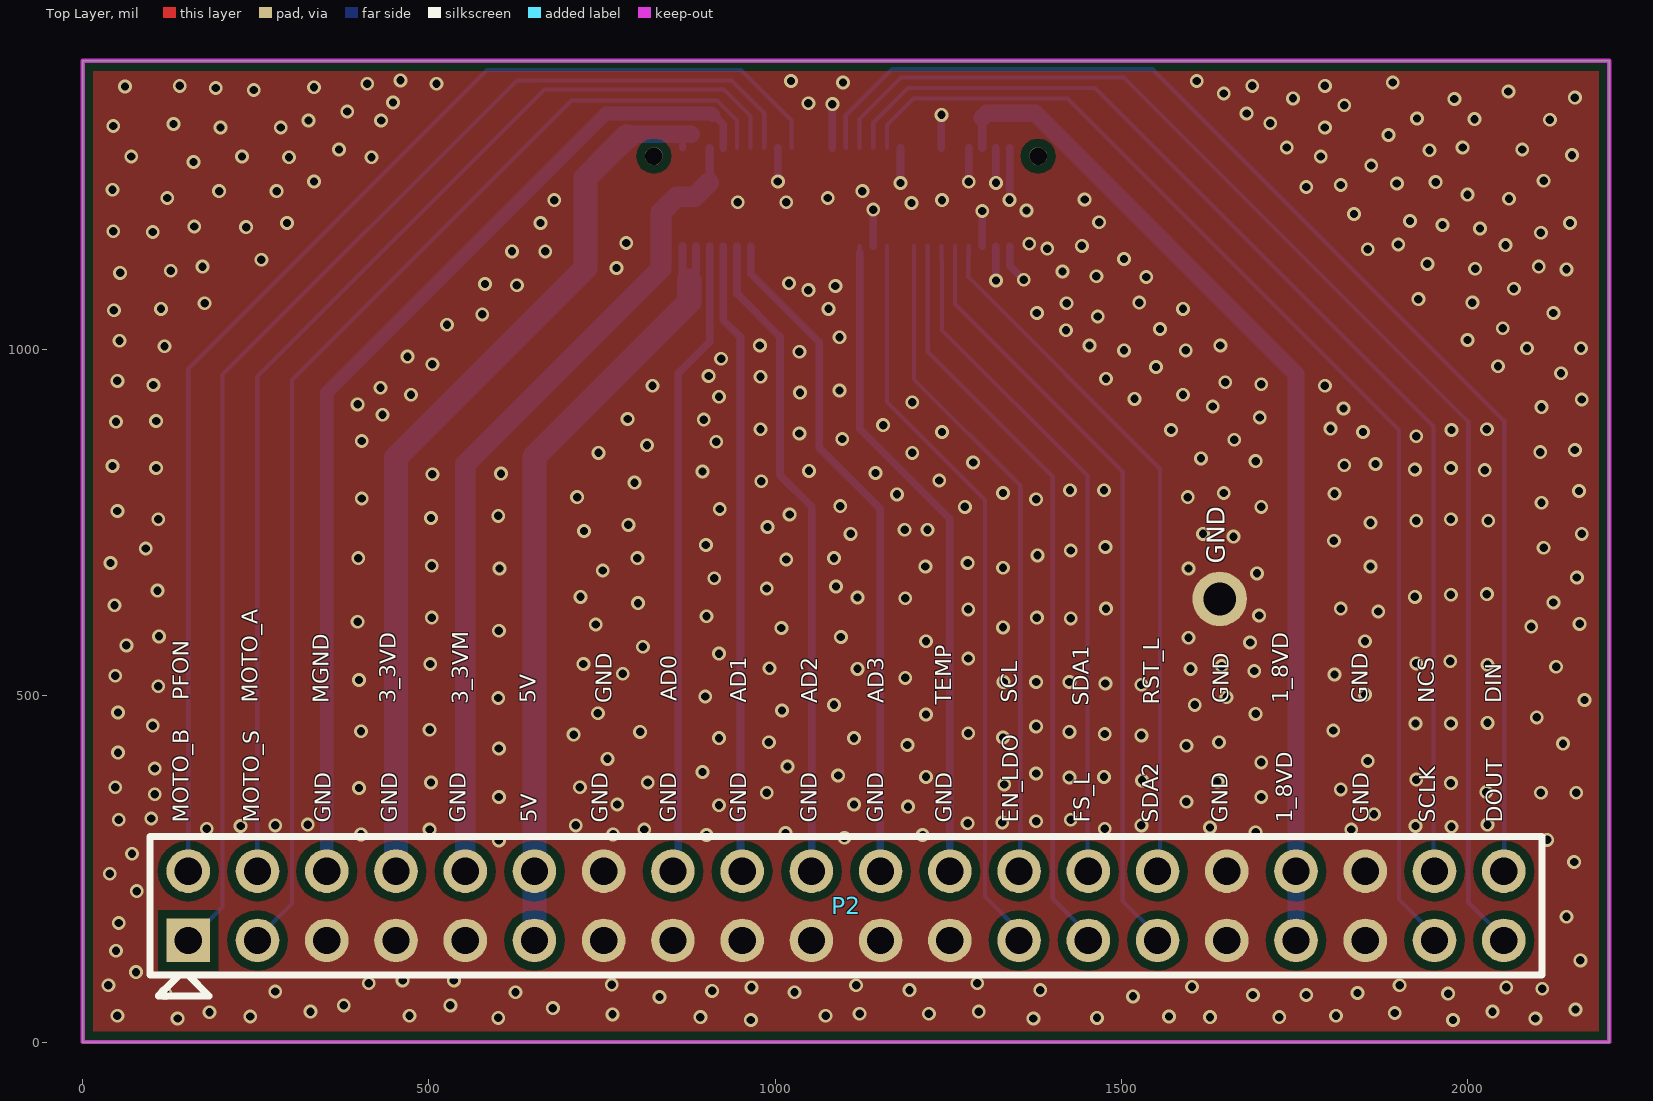
[diagram p0: Top Layer view]
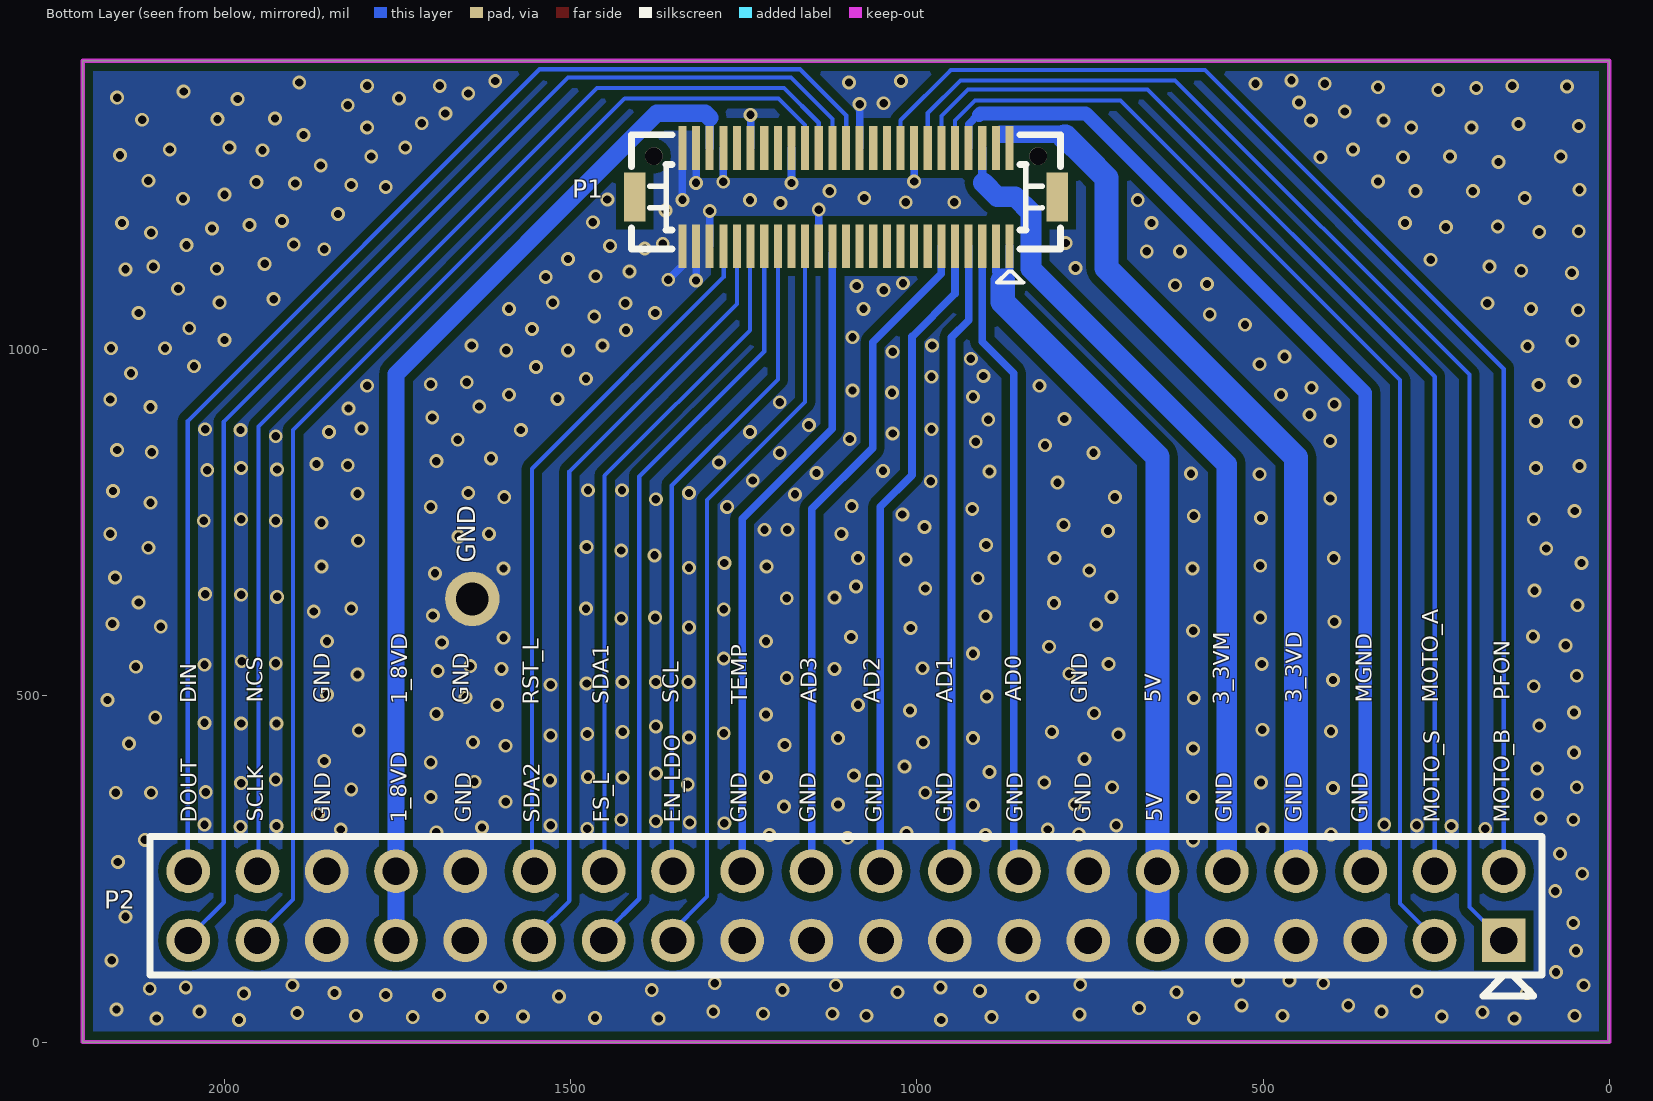
[diagram p1: Bottom Layer view, seen from below]
# Altium PCB MISC89329.PcbDoc
Units mil, origin at the board's own origin, x right, y up, seen from the top; angles counter-clockwise.
Board outline 2204.72 x 1417.32 mil, 2 copper layers (Top Layer, Bottom Layer); 2 components, 25 nets, 95 pads, 502 vias.

## Layer stack, top to bottom (the 12.6 mil dielectric is the usual default, probably not edited)
Top Layer: signal copper 1.4
Dielectric: dielectric 12.6, FR-4, Dk 4.8
Bottom Layer: signal copper 1.4

## Board outline
2204.72,1417.32 0,1417.32 0,0 2204.72,0

## Design rules (kind name [scope] priority, off if disabled: settings)
Clearance Clearance_1 [inpolygon] p1: gap=12
Clearance [All] p2: gap=6
DiffPairsRouting [All] p1: maxlimit=6 minlimit=6 mostfreqgap=6 maxuncoupledlength=500
HoleSize [All] p1: absolutevalues=TRUE maxlimit=500 minlimit=1 maxpercent=80.000 minpercent=20.000
HoleToHoleClearance [All] p1: gap=0 allowstackedmicrovias=TRUE
MinimumSolderMaskSliver [All] p1: minsoldermaskwidth=0
PlaneClearance [All] p1: clearance=6
PlaneConnect [All] p1: planeconnectstyle=Direct reliefexpansion=20 reliefentries=4 reliefconductorwidth=10 reliefairgap=10
PolygonConnect [All] p1: connectstyle=Direct reliefconductorwidth=10 reliefentries=4 polygonreliefangle="90 Angle"
RoutingVias [All] p1: holewidth=12 width=20 viastyle="Through Hole" minholewidth=12 minwidth=20 maxholewidth=12 maxwidth=20
SilkToSilkClearance [All] p1: silktosilkclearance=0
SilkscreenOverComponentPads [All] p1: minsilkscreentomaskgap=0
SolderMaskExpansion [All] p1: expansion=4
Width [All] p1: maxlimit=80 minlimit=6 preferedwidth=6 minimp=50.000000 maximp=50.000000 favimp=50.000000
20 further rules are at their usual default settings.

## Components (designator, comment, footprint, x,y, rotation, side; value= is the part's Value field where it differs from the comment)
P1 "#NAME?" CONN-SMD_DF12A-3.0-50DS-0.5 1102.36,1220.47 r180 bottom
P2 "#NAME?" HDR-TH_40P-P2.54-V-F-R2-C20-S2.54 1102.36,196.85 r0 top locked

## Footprints (in the part's own frame and the unit in brackets; to place one, negate y for a bottom-side part, rotate by r counter-clockwise, add the part's x,y. Pads: shape width x height; smd on the part's side, far side on the other; paste and mask are expansions set on the pad)
CONN-SMD_DF12A-3.0-50DS-0.5 [mm]
  round 0.65 hole 0.65 unplated: 0(-7.049,1.5) 0(7.049,1.5)
  rect 0.297x1.598 smd: 1(5.999,-1.798) 2(5.999,1.798) 3(5.499,-1.798) 4(5.499,1.798) 5(4.999,-1.798) 6(4.999,1.798) 7(4.499,-1.798) 8(4.499,1.798) 9(3.999,-1.798) 10(3.999,1.798) 11(3.499,-1.798) 12(3.499,1.798) 13(2.999,-1.798) 14(2.999,1.798) 15(2.499,-1.798) 16(2.499,1.798) 17(1.999,-1.798) 18(1.999,1.798) 19(1.499,-1.798) 20(1.499,1.798) 21(0.999,-1.798) 22(0.999,1.798) 23(0.499,-1.798) 24(0.499,1.798) 25(-0.001,-1.798) 26(-0.001,1.798) 27(-0.501,-1.798) 28(-0.501,1.798) 29(-1.001,-1.798) 30(-1.001,1.798) 31(-1.501,-1.798) 32(-1.501,1.798) 33(-2.001,-1.798) 34(-2.001,1.798) 35(-2.501,-1.798) 36(-2.501,1.798) 37(-3.001,-1.798) 38(-3.001,1.798) 39(-3.501,-1.798) 40(-3.501,1.798) 41(-4.001,-1.798) 42(-4.001,1.798) 43(-4.501,-1.798) 44(-4.501,1.798) 45(-5.001,-1.798) 46(-5.001,1.798) 47(-5.501,-1.798) 48(-5.501,1.798) 49(-6.001,-1.798) 50(-6.001,1.798)
  rect 0.798x1.796 smd: 51(-7.75,-0.003) 52(7.75,-0.003)
  silkscreen extent -7.87,-3.14 7.87,2.29
HDR-TH_40P-P2.54-V-F-R2-C20-S2.54 [mm]
  rect 1.6x1.6 hole 1: 1(-24.13,-1.27)
  round 1.6 hole 1: 2(-24.13,1.27) 3(-21.59,-1.27) 4(-21.59,1.27) 5(-19.05,-1.27) 6(-19.05,1.27) 7(-16.51,-1.27) 8(-16.51,1.27) 9(-13.97,-1.27) 10(-13.97,1.27) 11(-11.43,-1.27) 12(-11.43,1.27) 13(-8.89,-1.27) 14(-8.89,1.27) 15(-6.35,-1.27) 16(-6.35,1.27) 17(-3.81,-1.27) 18(-3.81,1.27) 19(-1.27,-1.27) 20(-1.27,1.27) 21(1.27,-1.27) 22(1.27,1.27) 23(3.81,-1.27) 24(3.81,1.27) 25(6.35,-1.27) 26(6.35,1.27) 27(8.89,-1.27) 28(8.89,1.27) 29(11.43,-1.27) 30(11.43,1.27) 31(13.97,-1.27) 32(13.97,1.27) 33(16.51,-1.27) 34(16.51,1.27) 35(19.05,-1.27) 36(19.05,1.27) 37(21.59,-1.27) 38(21.59,1.27) 39(24.13,-1.27) 40(24.13,1.27)
  silkscreen extent -25.53,-3.31 25.53,2.54

## Part data
P1: library part DF12A-50DS-0.5V(81)
P2: library part 2.54-2*20

## Free pads (board coordinates)
  round 78.74 hole 47.24: 0(1642,640)

## Via types
v1: diameter 20, hole 12, Top Layer to Bottom Layer, tented both sides, 502 vias

## Nets (pads, with @x,y where several pads share a name; then routed paths per layer and width w, separated by ;. In a path a pad name is that pad's centre, name@x,y a point inside that pad or via, vN(x,y) a via of type N, cw(c..) or ccw(c..) an arc to the next point about the centre after c; other vN are vias at no path point)
1_8VD: P1.46 P2.33 P2.34 | length 1470.2
  Bottom Layer w12: P1.46 1299.23,1328.77
  Bottom Layer w20: 1299.23,1331.51 1299.23,1333.23 1300.14,1334.14
  Bottom Layer w25: 1299.23,1335.05 1305.68,1341.5 1375.5,1341.5 1752.36,964.64 P2.34 P2.33
3_3VD: P1.2 P1.4 P2.8 | length 1327.6
  Bottom Layer w10: P1.2 P1.2@866.16,1311.84
  Bottom Layer w25: 794,1311 879,1311
  Bottom Layer w35: P2.8 452.36,844.36 726,1118 726,1248 755.5,1277.5 ; 771,1293 755.5,1277.5 ; 787,1307.5 785.5,1307.5 755.5,1277.5
3_3VM: P1.6 P2.10 | length 1205.4
  Bottom Layer w12: 905.53,1244.53 P1.6
  Bottom Layer w20: 903,1242 905.53,1244.53
  Bottom Layer w30: P2.10 552.36,834.36 835,1117 835,1198 858,1221 884,1221 904,1241
5V: P1.1 P1.3 P2.11 P2.12 | length 1149.9
  Bottom Layer w12: P1.1 866.16,1110.84 875,1102 ; 876,1103 885.85,1112.85 P1.3
  Bottom Layer w30: 875,1100 875,1102
  Bottom Layer w35: P2.11 P2.12 652.36,845.36 876,1069 876,1100
AD0: P1.5 P2.16 | length 901.5
  Bottom Layer w11: P2.16@860,267 860,966 905.53,1011.53 P1.5
AD1: P1.7 P2.18 | length 893.9
  Bottom Layer w11: P1.7 925.22,1042.78 950,1018 P2.18@950,266
AD2: P1.9 P2.20 | length 927.4
  Bottom Layer w11: 944.9,1095 P1.9 ; 945,1095 945,1081 1007,1019 1007,819 1053,773 P2.20@1053,267
AD3: P1.11 P2.22 | length 957.1
  Bottom Layer w11: P1.11@964.59,1128 P1.11 ; P1.11@965,1128 965,1110 1064,1011 1064,858 1152,770 P2.22@1152,270
DIN: P1.26 P2.40 | length 1942.1
  Bottom Layer w6: P1.26 1102,1291.66 1102,1338 1169,1405 1545,1405 2053,897 2053,356 ; P2.40@2053,259 2053,356 ; 2053,288 2053,356
DOUT: P1.28 P2.39 | length 1913.3
  Bottom Layer w6: P1.28 1122.07,1333.07 1182,1393 1504,1393 2001,896 2001,202 P2.39@2049,154
EN_LDO: P1.31 P2.25 | length 1076.1
  Bottom Layer w6: P1.31 1161.44,924.56 1303,783 1303,210 P2.25@1358,155
FS_L: P1.37 P2.27 | length 1085.3
  Bottom Layer w6: P1.37 1220.49,997.51 1401,817 1401,207 P2.27@1449,159
GND: P1.16 P1.24 P1.29 P1.34 P1.40 P1.44 P1.45 P1.47 P1.48 P1.49 P1.50 P2.5 P2.7 P2.9 P2.13 P2.14 P2.15 P2.17 P2.19 P2.21 P2.23 P2.31 P2.32 P2.35 P2.36 pad.0 | length 594
  Bottom Layer w11: v1(1003.96,1243.04) P1.16 ; P1.24 v1(1082.7,1354.7) ; P1.29 v1(1141.75,1202.25) ; v1(1181.12,1240.88) P1.34 ; P1.40 v1(1240.18,1339.18) ; v1(1279.55,1242.45) P1.44 ; P1.45 v1(1299.23,1200.23) ; v1(1318.92,1099.92) P1.47 ; v1(1318.92,1240.92) P1.48 ; P1.49 1338.6,1121.4 v1(1359,1101) ; v1(1338.6,1216.4) P1.50
  other v1: 965,32 1979,32 137,34 1373,34 2098,34 600,35 1465,35 892,36 1628,36 1728,36 242,37 1569,37 50,38 472,38 1073,38 1810,38 765,40 1122,41 1222,41 1895,42 183,43 329,44 1294,44 2036,44 2156,47 679,49 377,53 531,53 833,65 1517,66 1690,68 1767,68 1972,70 119,71 1841,71 625,72 1028,72 278,73 909,74 1194,75 1383,75 2108,77 966,79 2056,79 1602,80 37,82 1117,82 1902,82 764,83 413,85 1292,85 462,89 536,89 77,101 2163,118 48,132 52,172 2143,181 78,218 39,243 2154,260 71,272 601,291 2115,292 1100,295 901,299 1213,299 402,300 766,300 1015,302 1694,303 501,307 811,307 1832,307 179,308 1476,308 1628,310 1977,311 228,312 1925,312 278,313 712,313 1529,313 325,314 2029,314 1278,316 1328,317 1377,319 52,321 1427,321 99,323 1865,329 1192,340 919,342 772,343 1114,343 1594,347 601,354 1702,354 104,358 988,360 2106,360 2157,360 2027,361 1817,365 399,367 47,368 718,368 1331,372 1976,374 503,375 816,375 1639,376 1530,378 1926,379 1425,382 1218,383 1475,383 1091,385 1377,388 895,390 104,395 1018,398 1702,404 1856,406 758,409 51,418 601,424 1594,428 1191,429 2138,431 991,433 1641,433 919,439 1114,439 1329,440 1529,443 709,444 1476,445 1279,446 805,448 1425,448 402,449 1806,450 501,451 1377,456 101,457 1925,460 1976,460 2029,461 2100,469 1218,473 1694,474 744,475 51,476 1010,479 1085,487 1606,487 2169,494 600,497 1652,498 899,499 1852,502 109,514 1529,516 1477,518 1330,520 1377,520 1425,520 399,523 1188,526 47,529 1808,531 780,532 1692,536 1119,539 1600,539 992,540 2128,542 1645,543 2029,545 502,546 723,546 1926,547 1975,550 1279,554 919,561 809,571 63,573 1686,577 1218,579 1852,579 1597,584 1095,585 110,586 601,594 1009,598 1329,599 2092,600 741,603 2162,604 397,607 1427,612 504,613 1378,613 901,615 1699,616 1871,622 1279,625 1478,626 1817,626 46,631 802,634 2124,635 1188,641 1119,642 719,643 1924,643 1976,646 2028,647 108,652 988,655 1088,658 912,670 2158,671 1696,677 751,681 602,684 1597,684 1329,685 1217,687 1860,687 504,688 40,692 1278,692 1016,697 398,699 801,699 1085,699 1379,703 1427,710 91,713 2110,714 1477,715 900,718 1807,724 1662,730 1109,734 1618,734 2165,734 724,738 1187,740 1220,740 989,744 788,747 1860,750 1926,753 2030,753 109,755 1976,755 503,757 600,760 1021,762 50,767 920,770 1274,773 1702,773 1094,774 2107,779 1377,784 403,785 714,787 1596,787 1176,791 1808,792 1329,793 1648,793 2161,796 1426,797 1475,797 797,808 980,810 1237,811 505,820 604,821 1145,822 895,824 1049,825 2025,826 1924,827 106,829 1976,829 43,832 1822,833 1867,835 1286,837 1694,839 1615,843 745,851 1198,851 2105,852 2155,855 815,862 915,867 403,868 1663,870 1097,871 1926,875 1035,879 1241,881 1849,881 1572,884 1977,884 979,885 2028,885 1802,886 1156,891 48,896 106,897 897,899 787,900 1700,902 433,906 1821,915 2107,917 1632,918 397,921 1198,924 2165,928 1519,929 919,932 474,935 1589,935 1036,938 1093,941 430,945 823,948 1794,948 102,949 1702,950 1650,953 50,955 1478,958 979,961 904,962 2135,966 1550,975 2044,976 505,979 922,987 469,990 1035,997 1504,999 1593,999 2086,1002 2164,1002 118,1005 978,1006 1454,1006 1643,1006 53,1013 2000,1014 1093,1018 1420,1028 1556,1030 2051,1031 526,1036 1466,1048 577,1051 1378,1053 2124,1053 45,1057 113,1059 1077,1059 1589,1059 176,1067 1421,1067 1526,1068 2007,1068 1929,1073 1048,1086 2067,1088 1087,1092 627,1093 581,1095 1020,1096 1536,1105 1464,1106 54,1111 1415,1113 127,1114 2143,1116 2011,1117 771,1118 173,1120 2103,1120 1942,1124 258,1130 1504,1131 620,1142 668,1142 1856,1145 1393,1146 1443,1150 2055,1151 1900,1152 1367,1153 785,1154 2106,1169 101,1170 44,1171 2018,1175 236,1177 161,1178 1964,1180 295,1183 661,1183 2148,1183 1468,1184 1917,1186 1836,1196 1363,1201 1197,1212 946,1213 1016,1213 681,1216 1241,1216 1447,1217 2060,1218 122,1219 1076,1219 2000,1224 197,1229 280,1229 1126,1229 43,1231 1767,1235 1817,1238 1898,1240 1954,1242 334,1243 2110,1244 1861,1266 160,1271 298,1278 417,1278 70,1279 230,1279 1788,1279 2151,1281 1945,1288 370,1289 2079,1289 1739,1292 1993,1292 1886,1310 199,1321 286,1321 1794,1321 44,1323 131,1326 1715,1327 326,1331 431,1331 2119,1332 2010,1333 1927,1334 1681,1341 382,1344 1822,1353 1048,1356 448,1357 1981,1362 1748,1363 2155,1364 1648,1370 2059,1373 247,1375 192,1378 334,1379 61,1380 140,1381 1689,1381 1794,1381 411,1384 511,1384 1098,1386 1892,1386 1023,1388 1609,1388 459,1389
MGND: P1.8 P2.6 | length 1471.4
  Bottom Layer w11: 910.13,1339 912,1339 925.22,1325.78 P1.8
  Bottom Layer w20: P2.6 352.36,937.36 756,1341 908.13,1341 910.13,1339
MOTO_A: P1.12 P2.4 | length 1676.3
  Bottom Layer w6: P2.4@252,262 252,318 ; 252,287.35 252,318 ; P1.12 964.59,1337.41 926,1376 667,1376 252,961 252,318
MOTO_B: P1.14 P2.1 | length 1838.4
  Bottom Layer w6: P2.1@173,166 202,195 202,964 627,1389 937,1389 984.27,1341.73 P1.14
MOTO_S: P1.10 P2.3 | length 1673.2
  Bottom Layer w6: P2.3@263,161 302,200 302,956 706,1360 916,1360 944.9,1331.1 P1.10
NCS: P1.30 P2.38 | length 1730.1
  Bottom Layer w6: P1.30 1141.75,1327.75 1192,1378 1462,1378 1951,889 1951,317 ; P2.38@1951,251 1951,317 ; 1951,294 1951,317
PFON: P1.18 P2.2 | length 1845.8
  Bottom Layer w6: P2.2 152.36,972.36 584,1404 951,1404 1023.64,1331.36 P1.18
RST_L: P1.43 P2.30 | length 1001.4
  Bottom Layer w6: P1.43@1279,1135 1279,1105 1556,828 P2.30@1556,263 ; P1.43@1279.55,1135 P1.43
SCL: P1.35 P2.26 | length 948.1
  Bottom Layer w6: P1.35 1200.81,957.19 1354,804 P2.26@1354,265
SCLK: P1.32 P2.37 | length 1733
  Bottom Layer w6: P1.32 1161.44,1324.44 1200,1363 1422,1363 1901,884 1901,206 P2.37@1949,158
SDA1: P1.39 P2.28 | length 967.7
  Bottom Layer w6: P1.39@1240.18,1129 P1.39 ; P1.39@1241,1129 1241,1028 1451,818 P2.28@1451,269
SDA2: P1.41 P2.29 | length 1109.6
  Bottom Layer w6: P1.41@1259.86,1135 P1.41 ; P1.41@1260,1135 1260,1066 1502,824 1502,204 P2.29@1547,159
TEMP: P1.27 P2.24 | length 956.8
  Bottom Layer w6: P1.27@1122.07,1140 P1.27
  Bottom Layer w11: P1.27@1122,1140 1122,886 1252.36,755.64 P2.24
pads on no net: P1.0 P1.13 P1.15 P1.17 P1.19 P1.20 P1.21 P1.22 P1.23 P1.25 P1.33 P1.36 P1.38 P1.42 P1.51 P1.52

## Polygon pours and split planes (outlines as drawn)
GND on Bottom Layer "Bottom Layer-No Net" (solid, remove dead copper, pour order 1000): -106.73,1148.28 -76.73,1118.28 -76.73,-126.72 2310.27,-126.72 2374.27,-62.72 2388.27,-48.72 2389.27,-48.72 2389.27,1361.28 2291.27,1459.28 2130.27,1620.28 1664.27,1620.28 83.27,1620.28 0.27,1537.28 -106.73,1430.28 -106.73,1177.28
GND on Top Layer "Bottom Layer-No Net" (solid, remove dead copper, pour order 1001): -161,1202 -161,-21 -102,-80 -49,-133 14,-133 2309,-133 2353,-89 2382,-60 2382,-31 2382,1441 2275,1548 2134,1689 1602,1689 34,1689 -73,1582 -161,1494 -161,1211

## Keep-outs
Keep-Out Layer:
  the board outline again, w6

## Silkscreen, mask and mechanical layers (free items; w line width, h text height)
Top Overlay:
  text "GND" at 1658,691 h45 r90
  text "PFON" at 161,494 h40 r90
  text "AD0" at 866,492 h40 r90
  text "MOTO_A" at 261,490 h40 r90
  text "AD1" at 966,490 h40 r90
  text "SCL" at 1358,490 h40 r90
  text "MGND" at 363,489 h40 r90
  text "3_3VD" at 460,489 h40 r90
  text "5V" at 662,489 h40 r90
  text "GND" at 772,489 h40 r90
  text "AD2" at 1069,489 h40 r90
  text "AD3" at 1165,489 h40 r90
  text "GND" at 1663,489 h40 r90
  text "1_8VD" at 1749,489 h40 r90
  text "GND" at 1864,489 h40 r90
  text "NCS" at 1960,489 h40 r90
  text "DIN" at 2057,489 h40 r90
  text "3_3VM" at 565,488 h40 r90
  text "TEMP" at 1262,487 h40 r90
  text "RST_L" at 1563,487 h40 r90
  text "SDA1" at 1461,486 h40 r90
  text "MOTO_B" at 161,317 h40 r90
  text "MOTO_S" at 263,317 h40 r90
  text "GND" at 366,317 h40 r90
  text "GND" at 462,317 h40 r90
  text "GND" at 561,317 h40 r90
  text "5V" at 664,317 h40 r90
  text "GND" at 766,317 h40 r90
  text "GND" at 865,317 h40 r90
  text "GND" at 966,317 h40 r90
  text "GND" at 1068,317 h40 r90
  text "GND" at 1164,317 h40 r90
  text "GND" at 1263,317 h40 r90
  text "EN_LDO" at 1359,317 h40 r90
  text "FS_L" at 1462,317 h40 r90
  text "SDA2" at 1561,317 h40 r90
  text "GND" at 1662,317 h40 r90
  text "1_8VD" at 1755,317 h40 r90
  text "GND" at 1865,317 h40 r90
  text "SCLK" at 1961,317 h40 r90
  text "DOUT" at 2058,317 h40 r90
Bottom Overlay:
  text "GND" at 1629,692 h45 r270
  text "PFON" at 136,494 h40 r270
  text "AD0" at 841,492 h40 r270
  text "MOTO_A" at 239,490 h40 r270
  text "MGND" at 335,490 h40 r270
  text "3_3VD" at 436,490 h40 r270
  text "5V" at 640,490 h40 r270
  text "AD1" at 941,490 h40 r270
  text "NCS" at 1937,490 h40 r270
  text "GND" at 746,489 h40 r270
  text "AD2" at 1046,489 h40 r270
  text "AD3" at 1137,489 h40 r270
  text "SCL" at 1336,489 h40 r270
  text "GND" at 1639,489 h40 r270
  text "GND" at 1840,489 h40 r270
  text "DIN" at 2033,489 h40 r270
  text "TEMP" at 1237,488 h40 r270
  text "SDA1" at 1437,488 h40 r270
  text "1_8VD" at 1728,488 h40 r270
  text "3_3VM" at 541,487 h40 r270
  text "RST_L" at 1538,487 h40 r270
  text "5V" at 638,318 h40 r270
  text "SCLK" at 1936,318 h40 r270
  text "MOTO_B" at 136,317 h40 r270
  text "MOTO_S" at 237,317 h40 r270
  text "GND" at 341,317 h40 r270
  text "GND" at 436,317 h40 r270
  text "GND" at 537,317 h40 r270
  text "GND" at 741,317 h40 r270
  text "GND" at 839,317 h40 r270
  text "GND" at 941,317 h40 r270
  text "GND" at 1043,317 h40 r270
  text "GND" at 1138,317 h40 r270
  text "GND" at 1238,317 h40 r270
  text "EN_LDO" at 1334,317 h40 r270
  text "FS_L" at 1436,317 h40 r270
  text "SDA2" at 1537,317 h40 r270
  text "GND" at 1636,317 h40 r270
  text "1_8VD" at 1729,317 h40 r270
  text "GND" at 1839,317 h40 r270
  text "DOUT" at 2032,317 h40 r270